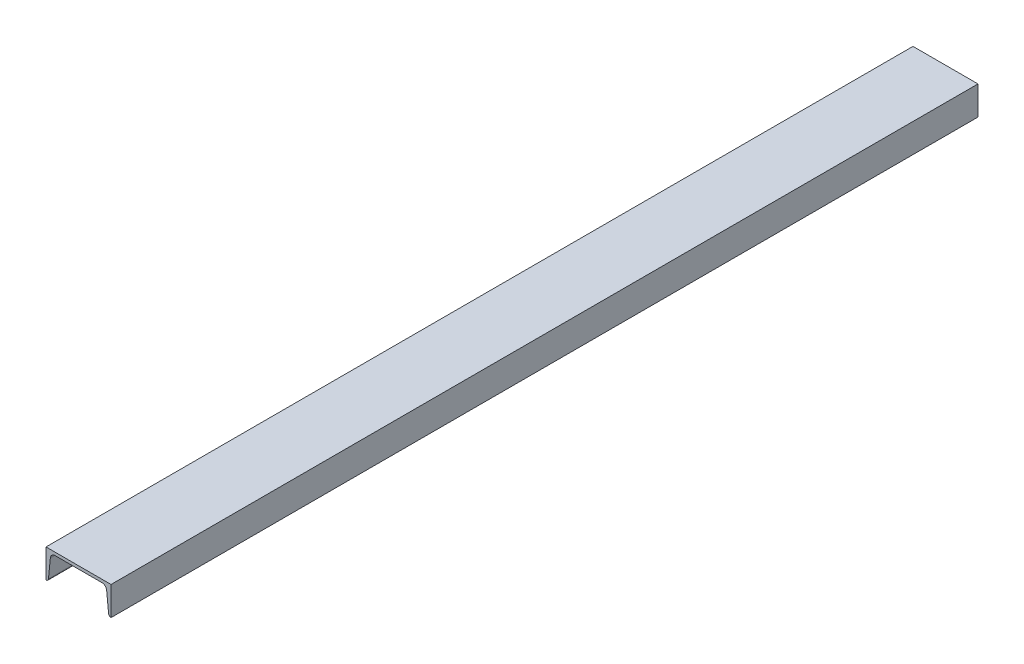
from build123d import *

# Parameters (mm, degrees)
BOSS_EXTRUDE_1_DEPTH = 800


with BuildPart() as part:
    # Sketch 1 → Boss-Extrude 1 (new, symmetric)
    with BuildSketch(Plane.XY):
        with BuildLine():
            Line((60, 0), (-60, 0))
            Line((-60, 0), (-60, -53))
            ThreePointArc((-60, -53), (-56.980458786, -51.836520772), (-55.522328009, -48.947720382))
            Line((-55.522328009, -48.947720382), (-51.988381432, -13.604559236))
            ThreePointArc((-51.988381432, -13.604559236), (-49.072119877, -7.826958457), (-43.03303745, -5.5))
            Line((-43.03303745, -5.5), (43.03303745, -5.5))
            ThreePointArc((43.03303745, -5.5), (49.072119877, -7.826958457), (51.988381432, -13.604559236))
            Line((51.988381432, -13.604559236), (55.522328009, -48.947720382))
            ThreePointArc((55.522328009, -48.947720382), (56.980458786, -51.836520772), (60, -53))
            Line((60, -53), (60, 0))
        make_face()
    extrude(amount=BOSS_EXTRUDE_1_DEPTH, both=True)


solid = part.part
